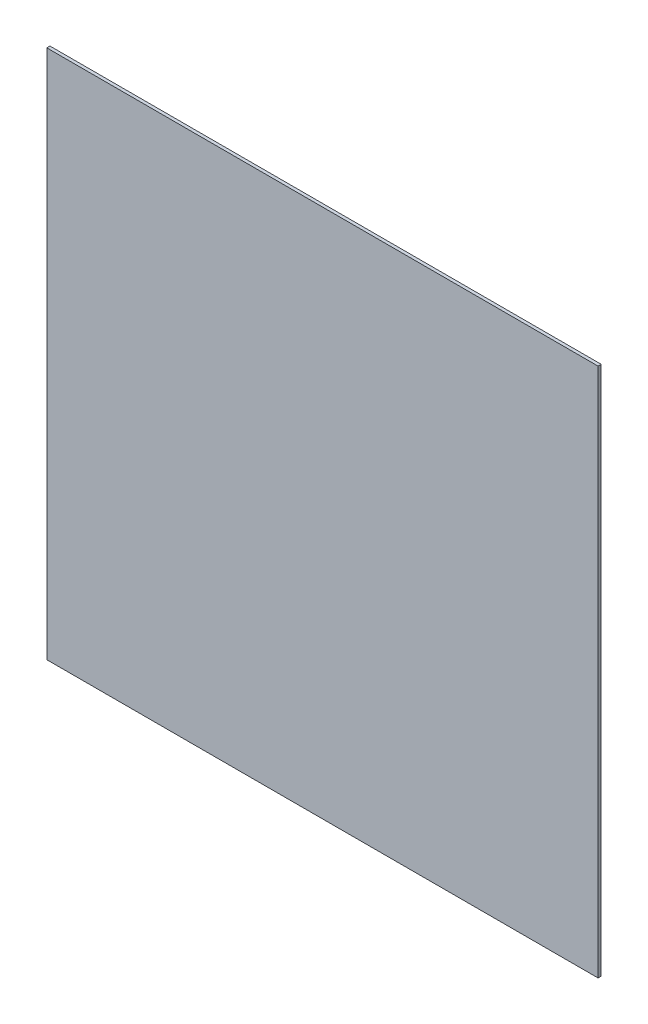
SolidWorks part; units mm, degrees
material "PMMA(有机玻璃)"
ref_plane "前视" through (0, 0, 0) normal (0, 0, 1) x (1, 0, 0)
ref_plane "上视" through (0, 0, 0) normal (0, 1, 0) x (1, 0, 0)
ref_plane "右视" through (0, 0, 0) normal (1, 0, 0) x (0, 0, -1)
sketch "草图1" plane through (0, 0, 0) normal (0, 0, 1) x (1, 0, 0)
  line L1 (-438, 421) -> (438, 421)
  line L2 (-438, 421) -> (-438, -421)
  line L3 (-438, -421) -> (438, -421)
  line L4 (438, 421) -> (438, -421)
  line L5 (-438, 421) -> (438, -421) construction
  line L6 (-438, -421) -> (438, 421) construction
  point P0 (0, 0)
  dimension "D1" = 842
  dimension "D2" = 876
extrude "凸台-拉伸1" add sketch "草图1" along normal blind 5
hole_wizard "M5 间隙孔1" positions "草图3" profile "草图2" hole size "M5" standard "GB"
sketch "草图3" plane through (0, 0, 5) normal (0, 0, 1) x (1, 0, 0)
  line L0 (-427.5, 273) -> (-427.5, -273) construction
  line L1 (-427.5, -273) -> (427.5, -273) construction
  line L2 (0, 273) -> (0, -273) construction
  line L3 (427.5, 273) -> (-427.5, 273) construction
  line L5 (-427.5, 0) -> (427.5, 0) construction
  line L6 (427.5, -273) -> (427.5, 273) construction
  point P0 (-375, -261)
  point P46 (415.5, 250)
  point P48 (-415.5, 250)
  point P58 (-125, -261)
  point P59 (125, -261)
  point P61 (-125, 261)
  point P62 (125, 261)
  point P64 (-375, 261)
  point P88 (375, -261)
  point P89 (375, 261)
  point P108 (415.5, 0)
  point P109 (-415.5, 0)
  point P110 (415.5, -250)
  point P111 (-415.5, -250)
  dimension "D1" = 12
  dimension "D2" = 12
  dimension "D5" = 3
  dimension "D3" = 12
  dimension "D6" = 4
  dimension "D4" = 2
sketch "草图2" plane through (-375, -261, 5) normal (1, 0, 0) x (0, -1, 0)
  line L0 (0, 0) -> (0, 5)
  line L1 (0, 5) -> (2.75, 5)
  line L2 (2.75, 5) -> (2.75, 0)
  line L5 (2.75, 0) -> (0, 0)
  line L11 (0, -6.35) -> (0, 107.95) construction
  dimension "通孔孔直径" = 5.5
  dimension "通孔孔深度" = 5
